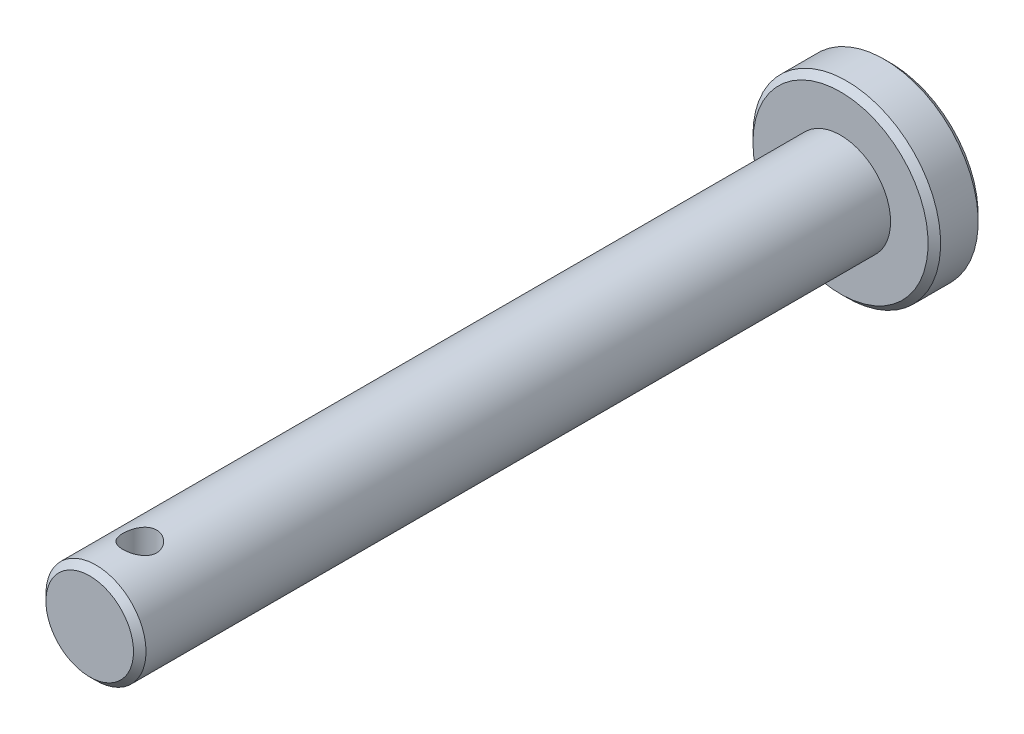
from build123d import *

# Parameters (mm, degrees)
SKETCH1_R               = 4
BOSS_EXTRUDE1_DEPTH     = 60
SKETCH2_R               = 7.5
BOSS_EXTRUDE2_DEPTH     = 4
CUT_EXTRUDE1_DEPTH      = 61.930288035
CUT_EXTRUDE1_DEPTH_BACK = 61.930288035
SKETCH3_R               = 1.35
CHAMFER1_SIZE           = 0.5


with BuildPart() as part:
    # Sketch1 → Boss-Extrude1 (new body)
    with BuildSketch(Plane.XY):
        Circle(SKETCH1_R)
    extrude(amount=BOSS_EXTRUDE1_DEPTH)

    # Sketch2 → Boss-Extrude2 (add)
    with BuildSketch(Plane(origin=(0, 0, 0), x_dir=(-1, 0, 0), z_dir=(0, 0, -1))):
        Circle(SKETCH2_R)
    extrude(amount=BOSS_EXTRUDE2_DEPTH)

    # Sketch3 → Cut-Extrude1 (cut, two sides: drawn at the far end of the back side and taken through both)
    with BuildSketch(Plane(origin=(0, 0, 0), x_dir=(1, 0, 0), z_dir=(0, 1, 0)).offset(-CUT_EXTRUDE1_DEPTH_BACK)):
        with Locations(Location((0, -56, 0), (0, 0, 270))):
            Circle(SKETCH3_R)
    extrude(amount=CUT_EXTRUDE1_DEPTH + CUT_EXTRUDE1_DEPTH_BACK, mode=Mode.SUBTRACT)

    # Chamfer1
    chamfer1_edges = [part.edges().sort_by_distance(p)[0] for p in [
        (-4, 0, 60),
        (7.5, 0, 0),
        (7.5, 0, -4),
    ]]
    chamfer(chamfer1_edges, length=CHAMFER1_SIZE)


solid = part.part
